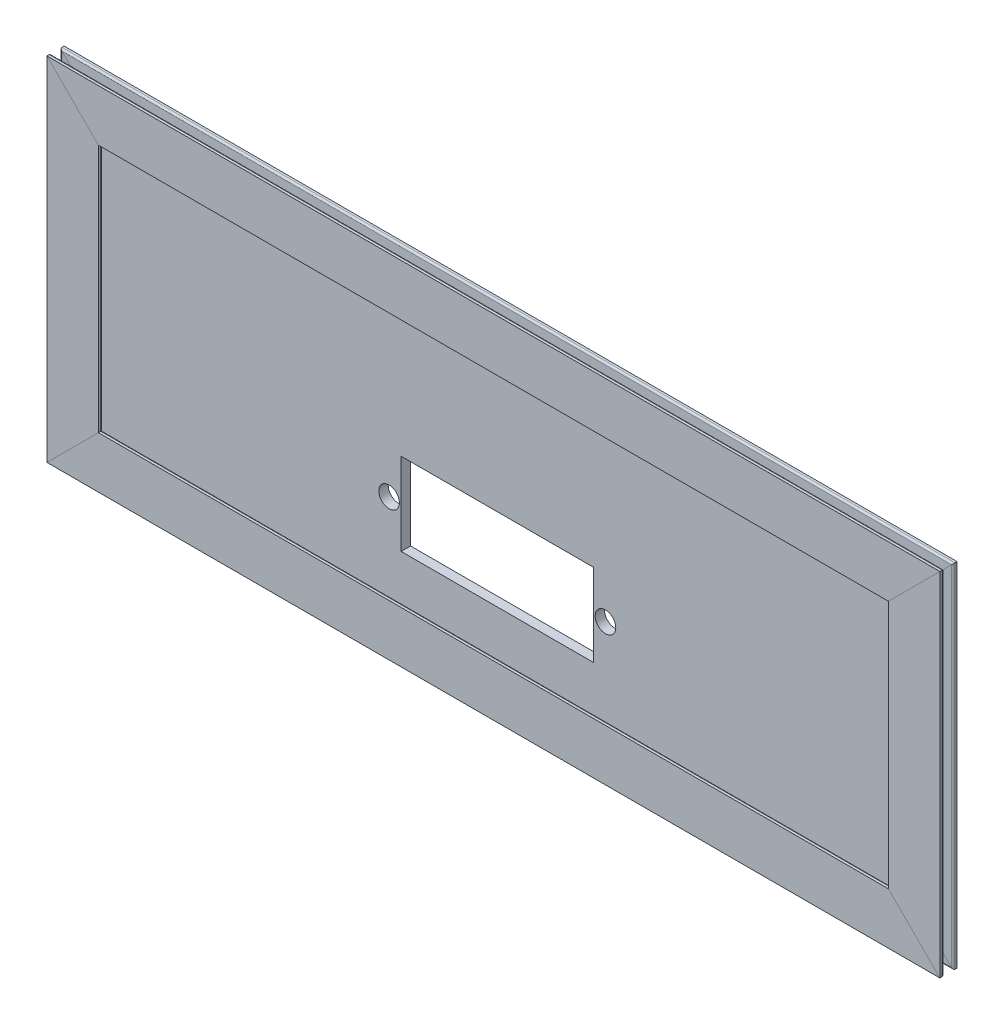
from build123d import *

# Parameters (mm, degrees)
ALUMINIUM_PROFILE_20_X_20_X_2_1_DEPTH      = 506.811388301
ALUMINIUM_PROFILE_20_X_20_X_2_1_DEPTH_BACK = 16.811388301
SKETCH1_W                                  = 6.2
SKETCH1_H                                  = 4.4
SKETCH1_ON_SEGMENT_2_W                     = 6.2
SKETCH1_ON_SEGMENT_2_H                     = 4.4
ALUMINIUM_PROFILE_20_X_20_X_2_1_2_DEPTH    = 208.622776602
SKETCH1_ON_SEGMENT_3_W                     = 6.2
SKETCH1_ON_SEGMENT_3_H                     = 4.4
ALUMINIUM_PROFILE_20_X_20_X_2_1_3_DEPTH    = 523.622776602
SKETCH1_ON_SEGMENT_4_W                     = 6.2
SKETCH1_ON_SEGMENT_4_H                     = 4.4
ALUMINIUM_PROFILE_20_X_20_X_2_1_4_DEPTH    = 208.622776602
SKETCH3_W                                  = 462
SKETCH3_H                                  = 147
BOSS_EXTRUDE1_DEPTH                        = 5.5
SKETCH4_R                                  = 6
SKETCH4_W                                  = 112
SKETCH4_H                                  = 48
CUT_EXTRUDE1_DEPTH                         = 280.582389467


with BuildPart() as part:
    # Sketch1 → Aluminium profile 20 X 20 X 2(1) (new, two sides: drawn at the far end of the back side and taken through both)
    with BuildSketch(Plane(origin=(-245, 87.5, 0), x_dir=(0, 1, 0), z_dir=(1, 0, 0)).offset(-ALUMINIUM_PROFILE_20_X_20_X_2_1_DEPTH_BACK)):
        with BuildLine():
            Line((4.5, 2.75), (14, 2.75))
            ThreePointArc((14, 2.75), (14.707106781, 3.042893219), (15, 3.75))
            Line((15, 3.75), (15, 5))
            Line((15, 5), (-15, 5))
            Line((-15, 5), (-15, 3.75))
            ThreePointArc((-15, 3.75), (-14.707106781, 3.042893219), (-14, 2.75))
            Line((-14, 2.75), (-4.5, 2.75))
            Line((-4.5, 2.75), (-4.5, -2.75))
            Line((-4.5, -2.75), (-14, -2.75))
            ThreePointArc((-14, -2.75), (-14.707106781, -3.042893219), (-15, -3.75))
            Line((-15, -3.75), (-15, -5))
            Line((-15, -5), (15, -5))
            Line((15, -5), (15, -3.75))
            ThreePointArc((15, -3.75), (14.707106781, -3.042893219), (14, -2.75))
            Line((14, -2.75), (4.5, -2.75))
            Line((4.5, -2.75), (4.5, 2.75))
        make_face()
        Rectangle(SKETCH1_W, SKETCH1_H, mode=Mode.SUBTRACT)
    extrude(amount=ALUMINIUM_PROFILE_20_X_20_X_2_1_DEPTH + ALUMINIUM_PROFILE_20_X_20_X_2_1_DEPTH_BACK)

    # Aluminium profile 20 X 20 X 2(1) mitre 1
    split(bisect_by=Plane(origin=(-245, 87.5, 0), x_dir=(-0.707106781, 0.707106781, 0), z_dir=(0.707106781, 0.707106781, 0)), keep=Keep.TOP)

    # Aluminium profile 20 X 20 X 2(1) mitre 2
    split(bisect_by=Plane(origin=(245, 87.5, 0), x_dir=(-0.707106781, -0.707106781, 0), z_dir=(-0.707106781, 0.707106781, 0)), keep=Keep.TOP)


with BuildPart() as body_2:
    # Sketch1 on segment 2 (carried to segment 2) → Aluminium profile 20 X 20 X 2_1 2 (new body)
    with BuildSketch(Plane(origin=(245, 104.311388301, 0), x_dir=(1, 0, 0), z_dir=(0, -1, 0))):
        with BuildLine():
            Line((4.5, 2.75), (14, 2.75))
            ThreePointArc((14, 2.75), (14.707106781, 3.042893219), (15, 3.75))
            Line((15, 3.75), (15, 5))
            Line((15, 5), (-15, 5))
            Line((-15, 5), (-15, 3.75))
            ThreePointArc((-15, 3.75), (-14.707106781, 3.042893219), (-14, 2.75))
            Line((-14, 2.75), (-4.5, 2.75))
            Line((-4.5, 2.75), (-4.5, -2.75))
            Line((-4.5, -2.75), (-14, -2.75))
            ThreePointArc((-14, -2.75), (-14.707106781, -3.042893219), (-15, -3.75))
            Line((-15, -3.75), (-15, -5))
            Line((-15, -5), (15, -5))
            Line((15, -5), (15, -3.75))
            ThreePointArc((15, -3.75), (14.707106781, -3.042893219), (14, -2.75))
            Line((14, -2.75), (4.5, -2.75))
            Line((4.5, -2.75), (4.5, 2.75))
        make_face()
        Rectangle(SKETCH1_ON_SEGMENT_2_W, SKETCH1_ON_SEGMENT_2_H, mode=Mode.SUBTRACT)
    extrude(amount=ALUMINIUM_PROFILE_20_X_20_X_2_1_2_DEPTH)

    # Aluminium profile 20 X 20 X 2_1 2 mitre
    split(bisect_by=Plane(origin=(245, -87.5, 0), x_dir=(-0.707106781, 0.707106781, 0), z_dir=(0.707106781, 0.707106781, 0)), keep=Keep.TOP)

    # Aluminium profile 20 X 20 X 2_1 2 mi 2
    split(bisect_by=Plane(origin=(245, 87.5, 0), x_dir=(0.707106781, 0.707106781, 0), z_dir=(0.707106781, -0.707106781, 0)), keep=Keep.TOP)


with BuildPart() as body_3:
    # Sketch1 on segment 3 (carried to segment 3) → Aluminium profile 20 X 20 X 2_1 3 (new body)
    with BuildSketch(Plane(origin=(261.811388301, -87.5, 0), x_dir=(0, -1, 0), z_dir=(-1, 0, 0))):
        with BuildLine():
            Line((4.5, 2.75), (14, 2.75))
            ThreePointArc((14, 2.75), (14.707106781, 3.042893219), (15, 3.75))
            Line((15, 3.75), (15, 5))
            Line((15, 5), (-15, 5))
            Line((-15, 5), (-15, 3.75))
            ThreePointArc((-15, 3.75), (-14.707106781, 3.042893219), (-14, 2.75))
            Line((-14, 2.75), (-4.5, 2.75))
            Line((-4.5, 2.75), (-4.5, -2.75))
            Line((-4.5, -2.75), (-14, -2.75))
            ThreePointArc((-14, -2.75), (-14.707106781, -3.042893219), (-15, -3.75))
            Line((-15, -3.75), (-15, -5))
            Line((-15, -5), (15, -5))
            Line((15, -5), (15, -3.75))
            ThreePointArc((15, -3.75), (14.707106781, -3.042893219), (14, -2.75))
            Line((14, -2.75), (4.5, -2.75))
            Line((4.5, -2.75), (4.5, 2.75))
        make_face()
        Rectangle(SKETCH1_ON_SEGMENT_3_W, SKETCH1_ON_SEGMENT_3_H, mode=Mode.SUBTRACT)
    extrude(amount=ALUMINIUM_PROFILE_20_X_20_X_2_1_3_DEPTH)

    # Aluminium profile 20 X 20 X 2_1 3 mitre
    split(bisect_by=Plane(origin=(-245, -87.5, 0), x_dir=(0.707106781, 0.707106781, 0), z_dir=(0.707106781, -0.707106781, 0)), keep=Keep.TOP)

    # Aluminium profile 20 X 20 X 2_1 3 mi 2
    split(bisect_by=Plane(origin=(245, -87.5, 0), x_dir=(0.707106781, -0.707106781, 0), z_dir=(-0.707106781, -0.707106781, 0)), keep=Keep.TOP)


with BuildPart() as body_4:
    # Sketch1 on segment 4 (carried to segment 4) → Aluminium profile 20 X 20 X 2_1 4 (new body)
    with BuildSketch(Plane(origin=(-245, -104.311388301, 0), x_dir=(-1, 0, 0), z_dir=(0, 1, 0))):
        with BuildLine():
            Line((4.5, 2.75), (14, 2.75))
            ThreePointArc((14, 2.75), (14.707106781, 3.042893219), (15, 3.75))
            Line((15, 3.75), (15, 5))
            Line((15, 5), (-15, 5))
            Line((-15, 5), (-15, 3.75))
            ThreePointArc((-15, 3.75), (-14.707106781, 3.042893219), (-14, 2.75))
            Line((-14, 2.75), (-4.5, 2.75))
            Line((-4.5, 2.75), (-4.5, -2.75))
            Line((-4.5, -2.75), (-14, -2.75))
            ThreePointArc((-14, -2.75), (-14.707106781, -3.042893219), (-15, -3.75))
            Line((-15, -3.75), (-15, -5))
            Line((-15, -5), (15, -5))
            Line((15, -5), (15, -3.75))
            ThreePointArc((15, -3.75), (14.707106781, -3.042893219), (14, -2.75))
            Line((14, -2.75), (4.5, -2.75))
            Line((4.5, -2.75), (4.5, 2.75))
        make_face()
        Rectangle(SKETCH1_ON_SEGMENT_4_W, SKETCH1_ON_SEGMENT_4_H, mode=Mode.SUBTRACT)
    extrude(amount=ALUMINIUM_PROFILE_20_X_20_X_2_1_4_DEPTH)

    # Aluminium profile 20 X 20 X 2_1 4 mitre
    split(bisect_by=Plane(origin=(-245, -87.5, 0), x_dir=(-0.707106781, -0.707106781, 0), z_dir=(-0.707106781, 0.707106781, 0)), keep=Keep.TOP)

    # Aluminium profile 20 X 20 X 2_1 4 mi 2
    split(bisect_by=Plane(origin=(-245, 87.5, 0), x_dir=(0.707106781, -0.707106781, 0), z_dir=(-0.707106781, -0.707106781, 0)), keep=Keep.TOP)


with BuildPart() as body_5:
    # Sketch3 → Boss-Extrude1 (new body)
    with BuildSketch(Plane.XY.offset(-2.75)):
        Rectangle(SKETCH3_W, SKETCH3_H)
    extrude(amount=BOSS_EXTRUDE1_DEPTH)

    # Sketch4 → Cut-Extrude1 (cut, through all)
    with BuildSketch(Plane(origin=(0, 0, -2.75), x_dir=(-1, 0, 0), z_dir=(0, 0, -1))):
        with Locations((-63, -22.5)):
            Circle(SKETCH4_R)
        with Locations((63, -22.5)):
            Circle(SKETCH4_R)
        with Locations((0, -22.5)):
            Rectangle(SKETCH4_W, SKETCH4_H)
    extrude(amount=-CUT_EXTRUDE1_DEPTH, mode=Mode.SUBTRACT)


solid = Compound([part.part, body_2.part, body_3.part, body_4.part, body_5.part])
